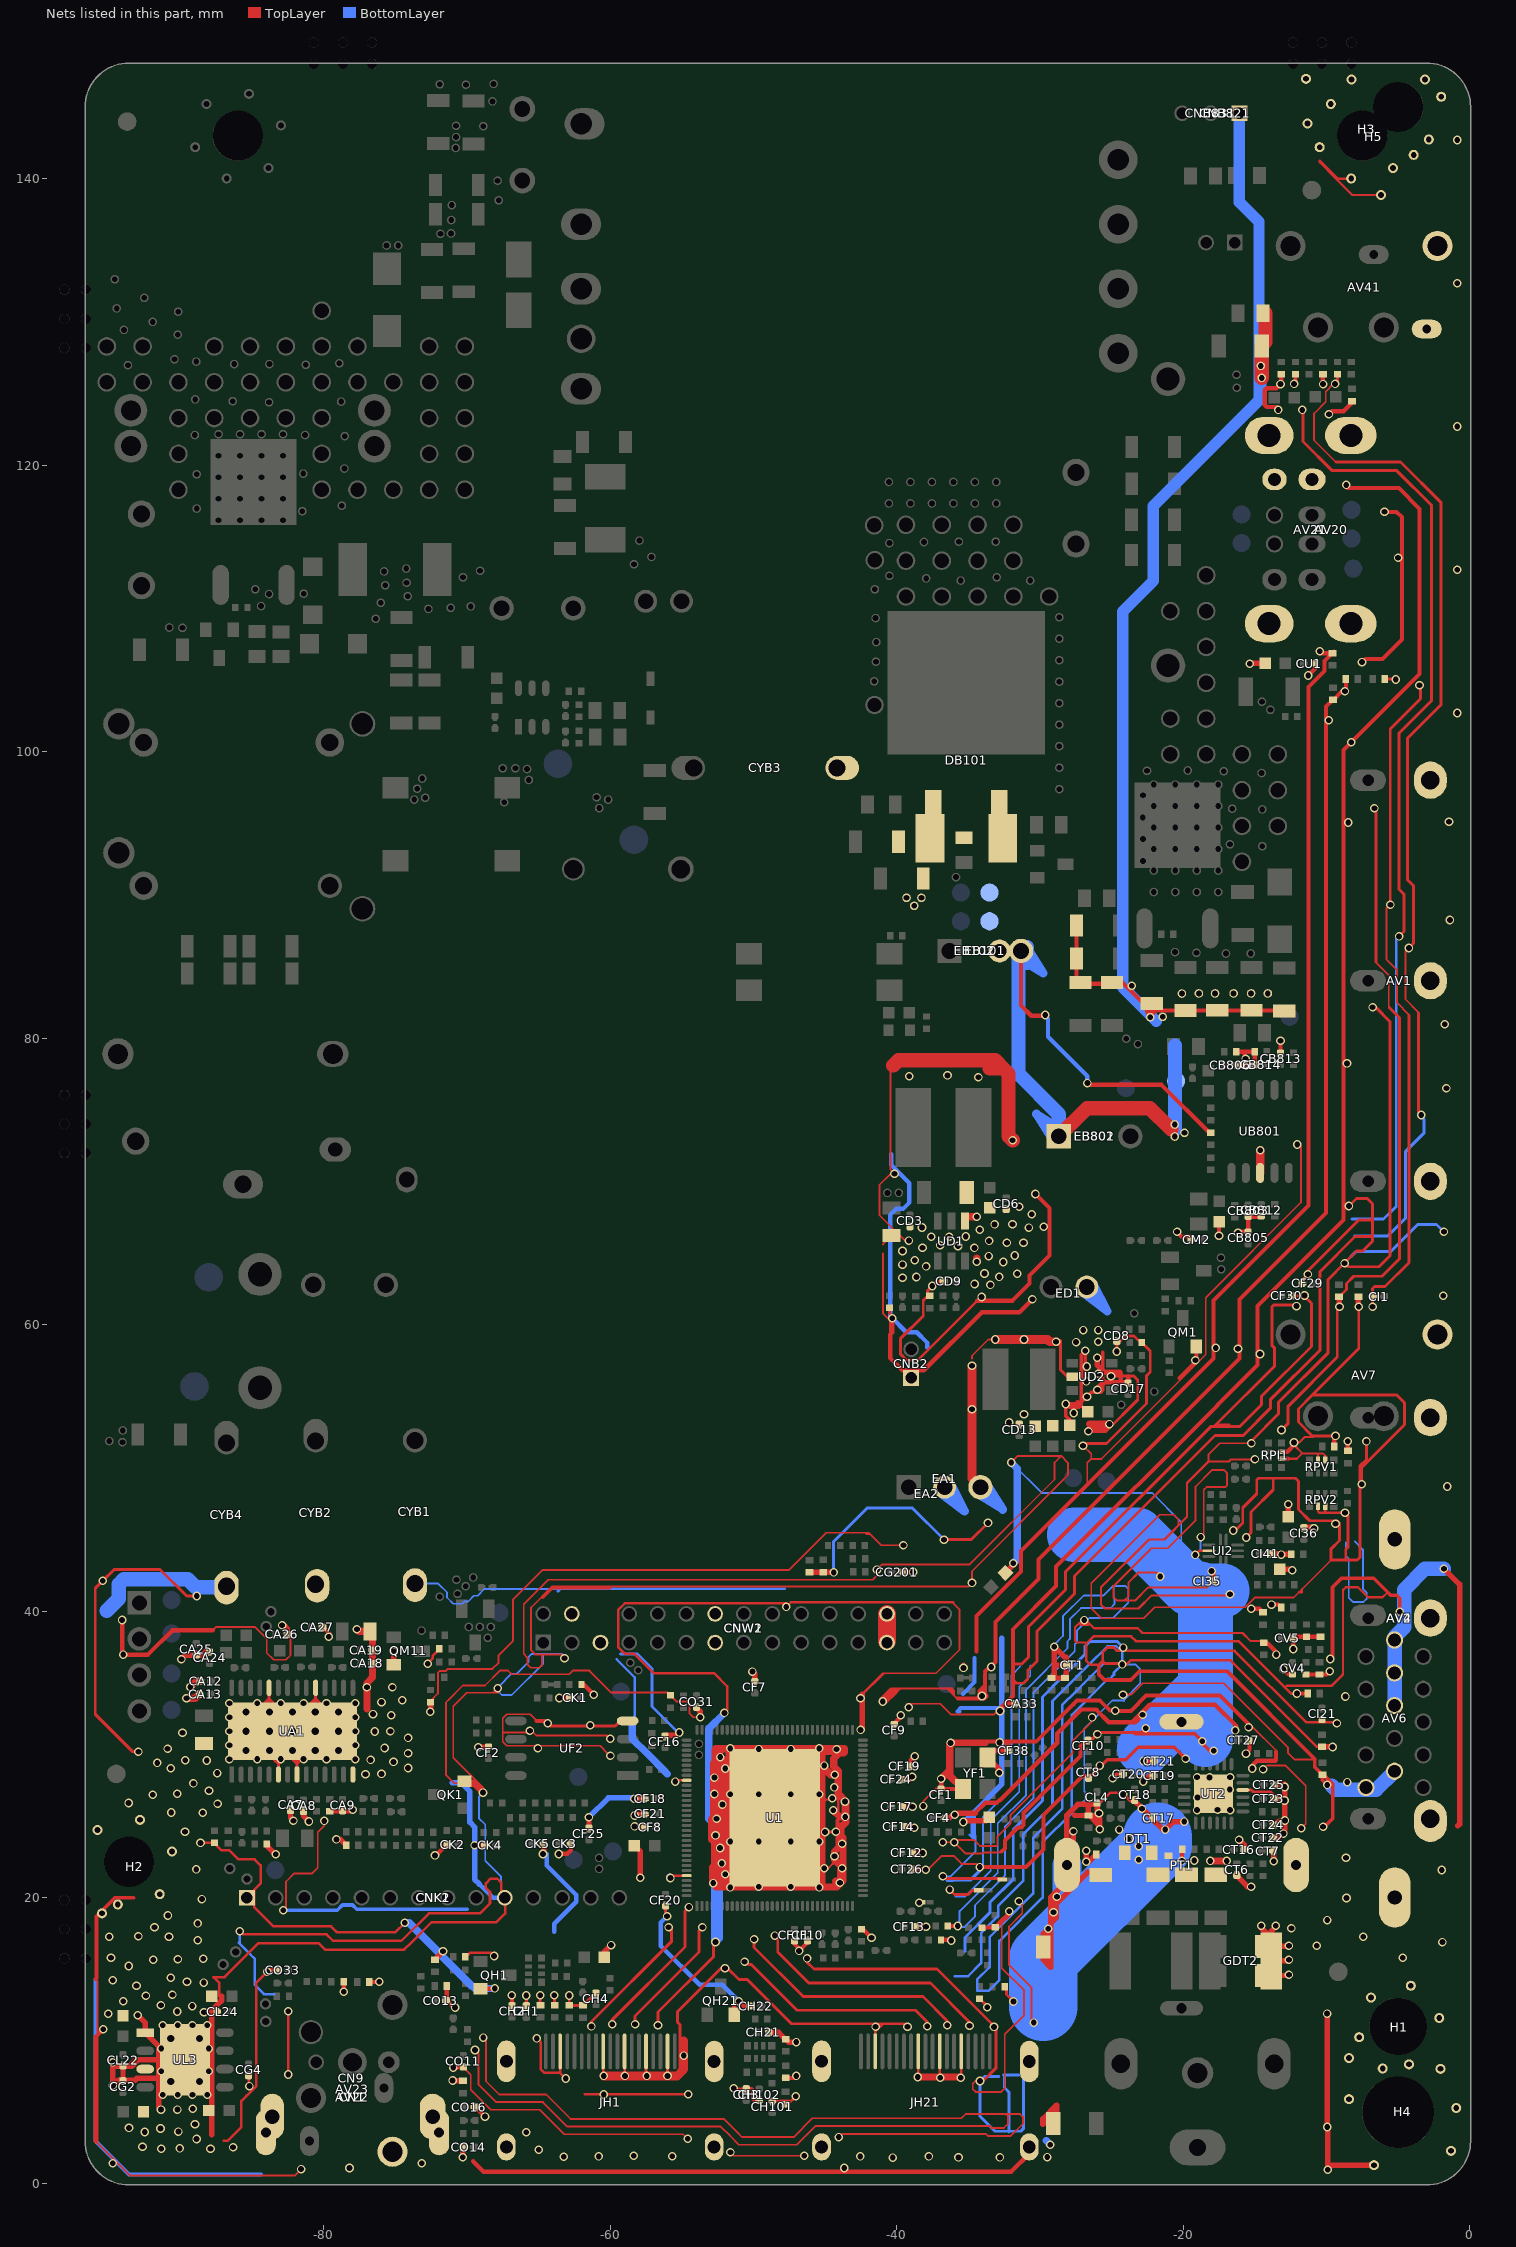
[diagram p0: the nets of this part, all layers, seen from the top]
# Altium PCB MISC86372.PcbDoc (part 9 of 16)
Units mm, origin at the board's own origin, x right, y up, seen from the top; angles counter-clockwise.
Board outline 96.73 x 148.13 mm, 2 copper layers (TopLayer, BottomLayer), stack 1.571 mm thick; 578 components, 318 nets, 2702 pads, 836 vias.

## Via types
v1: diameter 0.6, hole 0.4, TopLayer to BottomLayer, tented both sides, 816 vias
v2: diameter 0.7, hole 0.5, TopLayer to BottomLayer, tented both sides, 15 vias
v3: diameter 0.8, hole 0.5, TopLayer to BottomLayer, tented both sides, 5 vias

## Nets (pads, with @x,y where several pads share a name; then routed paths per layer and width w, separated by ;. In a path a pad name is that pad's centre, name@x,y a point inside that pad or via, vN(x,y) a via of type N, cw(c..) or ccw(c..) an arc to the next point about the centre after c; other vN are vias at no path point) (continued)
GND: (continued)
  TopLayer w0.203: v1(-92.943,30.175) -93.339,30.175 -95.953,32.79 -95.953,41.588 v1(-95.428,42.113) -94.634,42.907 -91.427,42.907 -89.566,41.046 v1(-88.875,41.046) ; UA1.EPAD@-84.277,33.426 -83.822,33.882 ; UA1.EPAD@-83.822,33.236 UA1.24@-83.822,34.661 ; -83.822,33.885 UA1.EPAD@-83.541,33.604 ; UA1.EPAD@-83.453,29.618 -83.172,29.337 ; UA1.6@-83.172,28.561 UA1.EPAD@-83.172,30.636 ; -83.172,29.34 UA1.EPAD@-82.716,29.796 ; UA1.EPAD@-82.153,29.618 -81.872,29.337 ; UA1.8@-81.872,28.561 UA1.EPAD@-81.872,29.964 ; -81.872,29.34 UA1.EPAD@-81.416,29.796 ; UA1.EPAD@-81.027,33.426 -80.572,33.882 ; UA1.EPAD@-80.572,33.28 UA1.19@-80.572,34.661 ; -80.572,33.885 UA1.EPAD@-80.291,33.604 ; CH1.2@-65.862,12.469 v1(-65.862,13.157) ; DH3.A@-64.897,12.495 v1(-64.897,13.183) ; -64.719,40.945 -64.072,41.593 ; v1(-64.364,32.156) -64.19,31.982 -62.357,31.982 ; -63.979,41.685 -64.072,41.593 ; v1(-63.906,13.183) -63.881,13.157 DH2.A@-63.881,12.49 ; v1@-62.865,13.047 v1(-62.865,13.157) DH81.A@-62.865,12.465 DH1.A@-61.906,12.465 DH1.A@-61.925,12.484 ; v1(-61.403,32.028) -61.449,31.982 -62.357,31.982 ; v1@-61.361,32.053 v1@-61.289,31.982 ; v1(-61.316,10.998) -61.316,11.341 -55.715,16.942 -55.715,17.912 -55.735,17.932 v1(-55.931,17.932) ; -59.999,41.593 -64.072,41.593 ; v1@-59.828,11.19 v1(-59.868,11.151) -59.868,11.46 -54.775,16.553 -54.775,19.063 v1(-54.508,19.329) ; -59.518,32.122 -59.657,31.982 -62.357,31.982 ; v1(-58.268,11.151) -58.268,11.731 -53.81,16.189 -53.81,17.678 v1(-53.569,17.919) ; v1@-56.629,11.112 v1(-56.667,11.074) -56.667,12.002 -52.782,15.888 -52.782,16.891 v1(-52.654,16.891) ; CF20.1@-56.138,19.388 -56.138,18.8 v1(-56.032,18.694) ; v1@-56,7.551 JH1.2@-56,9.258 ; -55.141,7.989 -55.141,11.122 -55.314,11.294 -55.314,12.026 -52.278,15.062 v1(-51.994,15.062) -51.807,15.062 -51.019,14.274 -50.437,14.274 -47.352,11.189 -42.139,11.189 ; v1(-51.381,6.688) -51.339,6.645 CH3.1@-50.588,6.645 ; v1(-50.622,15.508) -50.598,15.532 -50.545,15.532 -50.349,15.336 -50.17,15.336 -46.963,12.129 -38.699,12.128 -37.87,11.299 v1(-37.87,11.018) ; CH3.1@-50.506,6.669 -50.122,6.669 -50.057,6.604 -50.057,6.401 -50.053,6.397 -50.053,5.894 -49.957,5.798 CH102.1@-49.604,5.798 ; v1@-49.936,17.12 v1(-49.962,17.094) -49.962,16.511 -46.532,13.081 -38.167,13.081 -36.474,11.388 v1(-36.474,11.074) ; CH101.1@-48.819,5.81 -48.804,5.795 -48.142,5.795 -47.52,5.795 DH21.A@-47.738,5.577 ; v1(-48.509,17.34) -48.311,17.142 -48.311,16.189 -46.143,14.021 -37.652,14.021 -34.925,11.294 v1(-34.925,11.049) ; DH21.A@-47.904,5.557 -47.758,5.557 DH21.A@-47.738,5.577 ; DH21.A@-47.777,5.577 DH21.A@-47.738,5.577 ; v1(-47.05,6.133) -47.05,6.112 -47.585,5.577 DH21.A@-47.738,5.577 ; v1(-46.261,15.749) -46.279,15.731 -46.279,15.494 -45.783,14.999 -37.186,14.999 v1@-33.183,10.996 ; JH21.17@-41.5,9.258 -41.5,10.672 -40.983,11.189 -42.139,11.189 ; v1(-41.478,10.973) -41.262,11.189 ; RD5.1@-40.513,61.164 -40.513,60.782 -40.316,60.585 v1(-40.316,60.448) ; v1(-39.251,10.983) -39.456,11.189 -42.139,11.189 ; v1(-38.532,7.468) -38.5,7.499 JH21.11@-38.5,9.258 ; JH21.8@-37,9.258 -37,7.468 -37,7.46 v1(-36.957,7.417) ; CD9.1@-36.79,63.017 -37.186,63.017 v1(-37.516,62.687) -37.843,62.36 -37.843,61.995 -38.151,61.687 -38.151,60.604 -39.753,59.002 -39.753,57.963 -39.312,57.521 -38.523,57.521 -34.373,61.671 ; v1(-36.703,44.983) -34.798,44.983 v1(-33.63,46.152) ; v1@-36.662,21.605 v1(-36.779,21.488) -36.606,21.315 RA5.JP_2K@-32.63,21.315 ; v1@-36.424,11.1 v1@-36.424,11.269 ; v1(-36.297,20.553) -35.962,20.218 -35.013,20.218 -34.733,20.498 RA4.JP_2K@-34.28,20.498 ; v1@-35.535,7.366 -35.5,7.401 JH21.5@-35.5,9.258 ; RV5.1@-34.214,12.943 -33.68,12.41 v1(-33.68,12.344) ; v1(-34.188,7.188) -33.978,7.188 -33.058,8.108 ; -33.902,34.466 -33.927,34.466 -34.213,34.466 ; -33.864,35.179 -33.864,34.814 -33.902,34.776 -34.213,34.466 ; v1@-33.35,11.1 v1@-33.058,10.808 ; v1(-33.215,10.964) v1@-33.058,10.808 ; -33.058,8.153 v1@-33.058,10.808 ; RV3.1@-32.468,13.767 -32.339,13.638 -32.339,13.221 v1(-31.856,12.738) ; -31.902,35.204 -31.658,34.96 -31.153,34.96 -30.858,35.255 -30.858,35.844 -30.205,36.497 -30.205,38.592 -27.597,41.201 -27.597,42.445 -17.782,52.261 -15.813,52.261 -13.919,54.154 -13.919,54.747 -10.442,58.224 -10.442,63.707 -8.008,66.142 -7.645,66.142 ; -31.902,36.297 -31.268,36.297 -30.815,36.749 -30.815,38.883 -28.233,41.465 -28.233,42.715 -18.078,52.87 ; v1(-28.88,58.801) -28.578,58.499 ; -28.578,58.874 -28.578,56.842 -28.079,56.343 UD2.2@-27.74,56.343 ; v1(-27,51.537) -27,51.697 -25.366,51.697 -22.568,54.496 -22.568,56.426 -22.301,56.693 -22.301,58.159 RD8.2@-22.892,58.75 -22.98,58.75 -23.433,59.203 -24.051,59.203 -24.421,58.833 -24.638,58.833 v1@-24.638,58.141 ; v1(-26.619,52.553) -26.594,52.527 -25.399,52.527 -23.177,54.749 -23.177,56.128 -23.471,56.421 -24.361,56.421 -25.006,56.421 v1(-25.044,56.382) ; -25.705,55.666 -25.619,55.752 -25.474,55.896 ; v1(-25.155,53.051) v1@-24.874,53.051 ; -16.789,52.977 -17.741,52.977 ; v1(-16.51,45.618) -16.363,45.618 -15.845,46.136 -15.845,47.217 -14.869,48.192 -14.869,49.155 -14.756,49.268 -13.716,49.268 ; UT2.10@-15.832,27.504 -15.823,27.496 -15.227,27.496 -15.113,27.381 -14.356,27.381 -13.907,27.381 -13.625,27.099 CT23.1@-13.625,26.928 ; v1(-15.596,45.136) -15.261,45.471 -15.261,46.918 -13.716,48.463 -13.716,49.268 ; v1(-15.24,51.714) -15.24,51.866 -13.36,53.746 -13.36,54.547 -9.906,58.002 -9.906,63.119 v1(-8.738,64.287) ; v1(-13.142,52.638) -12.675,53.105 -12.675,54.299 -9.246,57.728 -9.246,61.138 v1@-9.119,61.265 ; CF30.2@-12.214,61.995 v1@-11.564,61.995 ; v1@-12.08,61.3 v1(-12.09,61.29) -12.09,61.366 -13.681,61.366 -13.818,61.23 -13.818,58.547 -13.615,58.344 -13.615,57.103 -17.741,52.977 ; CF29.2@-11.707,62.873 -11.707,63.096 v1(-11.294,63.509) -11.294,63.754 -7.742,67.305 -6.837,67.305 -6.782,67.361 ; v1(-11.684,123.85) -11.633,123.85 -11.633,121.642 -9.6,119.609 -5.093,119.609 -2.654,117.169 -2.654,103.569 -4.941,101.282 -4.941,90.387 -4.597,90.043 -4.597,87.431 v1(-4.932,87.096) ; v1(-11.532,62.027) v1@-11.564,61.995 ; v1@-10.251,125.669 v1(-10.236,125.654) ; -9.685,43.553 -7.856,43.553 -7.65,43.759 -7.65,50.135 -7.214,50.571 v1(-7.214,51.841) ; -9.673,43.566 -9.673,44.352 -9.096,44.929 -9.096,46.126 -9.271,46.302 -11.166,46.302 -11.95,47.085 -11.95,49.053 -12.165,49.268 -13.716,49.268 ; v1@-9.573,46.302 v1(-9.373,46.101) ; v1(-9.402,125.669) -9.298,125.669 -9.235,125.732 RA31.1@-9.235,126.346 ; v1(-9.373,52.222) -10.995,52.222 -11.963,53.191 -11.963,54.113 -10.983,55.093 ; -9.347,120.218 -4.841,120.218 ; DI2.A@-9.119,61.932 -8.606,62.444 -8.606,62.869 -8.103,63.373 -6.123,63.373 -4.902,64.594 -4.902,81.417 -5.613,82.128 ; v1(-8.707,46.853) -8.509,46.654 -8.509,44.446 -8.653,44.302 -8.653,44.281 -8.657,44.277 -8.657,43.553 ; v1(-8.433,68.275) -7.91,68.798 ; AV21.12@-8.3,122.07 AV21.12@-7.61,122.76 ; -7.849,66.142 -6.833,66.142 -6.782,66.192 ; v1(-7.747,61.239) -7.747,58.329 -10.983,55.093 ; v1(-7.544,48.844) -7.544,50.013 -4.547,53.01 -4.547,54.534 -5.105,55.093 -10.983,55.093 ; -7.417,68.798 -7.91,68.798 ; v1(-6.782,61.239) -6.775,61.246 CI1.2@-6.775,61.951 -6.782,61.957 -6.782,62.509 -6.636,62.655 -5.907,62.655 -4.242,64.32 -4.242,81.583 ; v1(-6.782,82.144) -6.563,82.144 -5.563,81.143 -5.563,64.795 -6.325,64.033 -8.484,64.033 v1(-8.738,64.287) ; v1(-6.655,96.037) -6.54,95.923 -6.54,85.324 ; DU1.A@-5.925,105.054 -5.182,105.054 v1(-5.156,105.029) ; -5.551,91.134 -5.551,91.415 ; v1(-5.537,89.306) -5.551,89.32 -5.551,91.415 ; -4.808,120.185 -4.841,120.218 ; v1(-4.247,86.287) -3.937,86.596 -3.937,90.642 -4.332,91.037 -4.332,100.958 -1.994,103.296 -1.994,117.371 -4.841,120.218 ; -3.581,81.748 -3.581,74.828 v1(-3.378,74.625) ; v1(-3.505,104.623) -3.429,104.546 -3.429,103.693 -5.551,101.571 -5.551,91.415 ; -34.404,33.934 -34.27,34.068 -34.27,34.122 -34.27,34.408 ; -34.404,33.934 -34.458,33.934 -35.806,33.934 -35.743,33.871 -34.521,33.871 -34.245,33.871 v1@-34.181,33.934 ; -34.404,33.934 v1@-34.181,33.934 ; -34.27,34.408 -34.127,34.265 -34.046,34.184 v1(-34.046,34.069) v1@-34.181,33.934 ; -34.27,34.408 -34.213,34.466 ; -18.078,52.87 -18.052,52.895 -17.822,52.895 -17.741,52.977 ; -18.078,52.87 -16.066,52.87 -14.529,54.407 -14.529,54.999 -11.051,58.476 -11.051,61.482 v1@-11.564,61.995 ; v1(-8.738,64.287) -7.899,65.126 -7.467,65.126 -6.782,65.811 -6.782,66.192 ; -7.91,68.798 -7.152,68.798 -6.782,68.428 -6.782,67.361 ; -6.782,66.192 -6.782,67.361
  TopLayer w0.229: v1@-60.5,7.589 v1@-60.5,7.592 ; v1@-57.5,7.589 JH1.5@-57.5,9.258 ; CT10.2@-26.645,31.007 -26.385,31.007 v1(-25.99,31.401) -25.868,31.524 -23.419,31.524 -22.915,31.524 v1(-22.619,31.82) ; v1@-25.808,29.112 -25.303,29.616 ; v1(-24.932,28.325) -24.932,28.366 -24.698,28.6 CT20.2@-24.254,28.6 ; -24.663,29.616 -25.303,29.616 ; -20.058,29.913 -20.631,30.486 -23.153,30.486 -24.023,29.616 -25.303,29.616 ; UT2.10@-15.832,27.504 UT2.10@-15.815,27.521
  TopLayer w0.254: -95.94,14.301 -95.869,14.372 -95.869,18.69 -94.576,19.983 -93.278,19.983 ; DH1.A@-61.906,12.465 -61.894,12.465 CH4.1@-61.006,13.353 ; CF5.1@-60.406,16.038 CF5.1@-60.406,15.824 CF5.1@-60.406,16.2 ; v1(-39.726,32.715) -39.726,32.562 CF9.1@-40.174,32.114 -40.174,32.191 v1@-39.675,32.69 ; CF1.1@-36.687,27.577 YF1.2@-35.369,27.577 ; CD10.1@-27.911,53.329 -28.194,53.612 v1(-28.194,54.454) ; -27.381,54.61 -27.33,54.559 -27.178,54.559 -27.178,54.305 -27.254,54.229 -27.969,54.229 v1(-28.194,54.454) ; -27.112,54.304 -27.112,54.574 ; v1(-26.764,56.027) -26.848,56.11 v1(-26.848,58.161) -27.112,57.897 -27.112,54.574 ; v1@-26.111,31.547 -26.111,31.54 v1@-26.094,31.558 ; -25.911,36.093 -25.911,35.603 -25.493,35.185 -23.666,35.185 -23.045,35.806 -16.95,35.806 -10.82,29.676 -10.82,29.114 -10.287,28.58 DV4.A@-10.287,28.556 ; -25.852,36.241 -25.616,36.477 ; -25.73,55.265 -26.421,55.265 v1(-26.72,54.966) -27.112,54.574 ; -25.619,55.417 -25.619,55.752 -25.619,55.859 -25.619,55.913 -25.619,56.772 -25.619,58.045 ; v1@-24.079,27.102 v1(-24.181,27.203) -24.152,27.203 -23.701,26.753 CT18.2@-23.393,26.753 ; -23.419,31.524 -23.334,31.439 -19.196,31.439 v1(-18.673,30.916) -18.83,30.916 -18.157,30.243 v1(-17.862,30.243) ; -20.058,29.913 v1(-19.837,29.693) ; v1(-13.032,35.954) -12.644,35.567 CV4.1@-12.37,35.567 ; RV6.1@-11.43,35.567 DV6.A@-10.49,35.567 -9.983,35.567 v1(-9.763,35.787) ; v1(-10.236,24.942) -10.135,24.942 -9.55,25.527 -9.55,27.897 -10.21,28.556 DV4.A@-10.287,28.556 ; v1(-9.946,27.858) -10.287,28.199 DV4.A@-10.287,28.556 ; v1(-9.728,36.652) -9.576,36.805 -9.576,41.665 -8.95,42.291 -6.706,42.291 -5.728,41.313 -5.524,41.11 -5.093,41.11 -4.877,40.894 v1(-4.877,39.954) ; AV6.16@-5.446,20 AV6.16@-5.227,20 ; v1(-28.194,54.454) -27.232,54.454 -27.112,54.574
  TopLayer w0.279: CF17.1@-39.58,26.34 -38.911,26.34 v1(-38.903,26.332) ; v1(-36.241,30.794) -36.161,30.874 -35.952,30.874 ; v1(-35.338,36.03) v1@-35.338,36.256 ; -34.417,37.177 -34.417,39.646 -31.319,42.744 -31.319,44.195 -27.331,48.183 ; v1(-34.215,22.123) -33.477,22.123 ; v1@-33.96,22.123 -33.477,22.123 ; -33.826,35.777 -33.51,36.092 v1@-33.459,36.092 ; v1@-33.495,36.056 v1@-33.459,36.092 ; v1@-33.403,36.092 v1@-33.459,36.092 ; v1(-32.821,30.819) v1@-32.876,30.874 ; v1(-32.791,33.02) -32.791,33.066 -32.33,33.528 ; v1@-32.756,33.229 -32.457,33.528 ; -32.672,23.216 -32.451,23.436 -32.451,23.98 -31.537,24.894 -31.294,24.894 ; -31.902,34.661 -31.902,34.309 ; CA33.1@-31.573,33.528 -32.33,33.528 ; -31.519,24.851 -31.475,24.894 -31.294,24.894 ; v1(-28.999,37.503) -28.956,37.46 DK3.A@-28.956,35.421 ; -27.675,33.475 -27.792,33.358 ; -27.318,48.196 -26.703,48.81 -17.889,57.625 v1@-17.889,58.42 ; CT10.2@-26.645,30.832 -26.916,30.832 -27.18,30.568 -27.18,29.869 -31.14,25.908 -31.14,25.048 -31.294,24.894 ; v1(-25.832,29.21) -25.808,29.186 -25.808,29.112 -26.442,28.478 CT8.1@-26.619,28.478 -27.027,28.478 -29.743,25.761 -29.743,23.361 -30.981,22.123 -33.477,22.123 ; v1@-24.689,33.02 -24.028,33.02 ; v1(-20.429,66.469) -20.141,66.181 -20.141,66.139 -19.478,66.139 CM2.1@-19.478,65.913 ; -20.26,56.267 -19.152,57.375 v1(-19.152,57.506) -19.088,57.569 QM1.E@-19.088,58.471 ; v1(-17.726,58.369) -17.838,58.369 v1@-17.889,58.42 ; -17.621,54.354 -28.881,43.094 -28.881,41.734 -31.902,38.712 -31.902,36.297 -31.902,35.204 -31.902,34.309 ; -17.607,54.368 -14.8,57.174 -14.8,59.106 ; v1(-16.18,58.318) v1@-16.078,58.42 ; v1(-15.439,31.885) -15.439,32.102 -17.424,34.087 -22.588,34.087 -23.655,33.02 -24.028,33.02 ; v1(-14.64,57.94) -14.8,58.101 -14.8,59.106 ; v1(-9.834,102.184) v1@-10.033,102.384 ; DU4.A@-9.459,106.985 -10.135,106.308 -10.135,105.613 -11.252,104.496 -11.252,68.3 -17.889,61.663 v1@-17.889,58.42 ; DU2.A@-8.655,105.054 -8.655,104.274 v1(-8.712,104.216) -8.92,104.216 -9.523,103.613 DU3.A@-9.55,103.613 -10.033,103.131 v1@-10.033,102.384 ; v1(-8.611,118.618) -8.534,118.542 -8.534,118.39 -4.947,118.39 -3.505,116.948 -3.505,105.423 v1(-8.28,100.648) -8.814,100.115 -8.814,67.29 -14.8,61.304 -14.8,59.106 ; v1(-7.518,106.248) -7.29,106.477 -6.08,106.477 -4.724,107.832 -4.724,116.36 -5.106,116.741 v1(-5.95,116.741) ; -35.952,30.874 -33.63,30.874 ; -35.952,30.874 -36.16,30.666 -36.16,30.577 -36.019,30.718 -33.785,30.718 -33.63,30.874 ; -33.63,30.874 v1@-32.876,30.874 ; v1@-33.459,36.092 -33.122,36.43 -33.122,39.217 -30.1,42.239 -30.1,43.599 -16.078,57.621 v1@-16.078,58.42 ; v1@-32.876,30.874 -30.277,30.874 -27.792,33.358 ; -32.457,33.528 -31.902,34.082 -31.902,34.309 ; -32.457,33.528 -32.33,33.528 ; -27.792,33.358 -27.406,33.744 -25.828,33.744 -25.13,33.045 v1(-24.74,33.045) -24.714,33.02 -24.028,33.02 ; v1@-16.078,58.42 -16.078,61.75 -10.033,67.795 v1@-10.033,102.384
  TopLayer w0.3: EB101.2@-31.323,86.081 -31.323,82.275 -30.607,81.559 v1@-29.642,81.559 ; RB822.2@-27.459,87.859 RB821.2@-27.459,85.547 -27.459,84.077 -27.178,83.796 -24.867,83.796 -24.79,83.872 -24.245,83.872 -22.291,81.918 -22.271,81.918 -13.06,81.918 RB818.2@-13.03,81.888 ; v1(-26.692,76.857) -26.568,76.733 -24.663,76.733 ; v1@-26.518,76.733 -24.663,76.733 ; RB134.1@-18.085,73.399 -18.182,73.399 -21.516,76.733 -24.663,76.733 ; v1(-17.501,66.192) CB801.2@-17.501,67.188 ; CB806.2@-16.41,78.105 -16.235,78.105 -15.248,78.105 CB814.2@-15.223,78.13 ; RB803.1@-16.231,79.045 -15.729,79.045 ; v1(-16.18,66.396) -16.106,66.469 CB805.1@-15.469,66.469 CB803.2@-15.469,67.52 CB812.1@-14.58,67.52 ; v1(-15.646,78.562) -15.729,78.645 -15.729,79.045 ; RB833.1@-15.223,79.041 -15.227,79.045 -15.729,79.045 ; CB814.2@-15.005,78.13 RB833.1@-15.005,79.045 ; CB813.1@-13.208,78.812 v1@-13.208,79.807 ; v1@-10.251,125.669 DA31.A@-10.251,126.346
  TopLayer w0.305: -95.91,2.989 -95.91,10.287 v1(-95.402,10.795) ; v1(-94.082,39.37) -94.082,37.033 v1(-94.005,36.957) -92.278,36.957 -90.588,38.648 -87.757,38.648 ; v1(-83.957,14.808) -83.83,14.935 CO33.1@-83.28,14.935 ; v1(-82.912,39.01) -82.732,39.01 -82.502,38.78 CA26.1@-82.502,38.372 ; CA27.2@-80.038,38.869 -79.603,38.434 -79.603,38.253 v1(-79.654,38.202) ; RA11.1@-79.668,26.023 RA11.1@-79.588,26.023 ; RA11.1@-79.582,26.018 CA9.1@-78.677,26.018 ; RO4.1@-78.62,14.118 -78.62,13.418 v1(-78.613,13.411) ; v1(-77.987,26.119) -78.083,26.023 CA9.1@-78.689,26.023 -78.04,26.023 v1@-77.978,26.086 ; DI9.A@-76.816,14.101 -76.145,14.101 v1(-76.124,14.122) ; v1(-72.238,22.936) -72.177,22.936 CK2.1@-71.425,23.688 ; DI6.A@-71.406,13.818 CO13.1@-71.406,12.802 -70.929,12.324 v1(-70.835,12.324) ; v1(-70.968,8.128) -70.961,8.135 CO11.1@-70.256,8.135 ; -69.571,1.575 -68.847,0.851 -32.017,0.851 -30.75,2.118 JH21.23@-30.75,2.59 ; CO16.1@-69.425,5.371 -68.76,4.705 v1(-68.747,4.705) ; v1(-69.215,30.496) -69.197,30.514 CF2.1@-68.504,30.514 ; QH1.E@-69.063,13.627 -68.089,13.627 v1(-68.062,13.654) ; v1(-66.878,13.176) -66.861,13.158 CH2.2@-66.861,12.474 ; -65.134,32.325 -64.618,32.325 -64.449,32.156 v1(-64.364,32.156) ; v1(-63.602,23.038) -63.593,23.047 -63.009,23.047 -62.745,23.31 CK3.1@-62.745,23.749 ; RF13.2@-62.008,34.87 -61.852,34.87 -61.159,34.177 v1(-61.159,34.161) ; QH21.E@-51.333,11.811 -51.333,12.476 v1@-51.046,12.763 ; v1(-51.033,12.763) v1@-51.046,12.763 ; CH22.2@-50.078,12.421 -50.704,12.421 v1@-51.046,12.763 ; DH22.A@-47.904,7.38 DH22.A@-47.611,7.38 ; DH22.A@-47.752,7.403 -47.157,7.403 v1(-47.015,7.544) ; CF11.2@-47.14,16.95 -47.14,16.762 -46.821,16.442 v1(-46.821,16.273) -46.226,16.867 CF10.1@-46.226,16.95 ; RF16.2@-42.469,17.799 -42.368,17.799 v1(-41.766,17.197) ; v1(-40.316,60.448) -40.316,59.445 -40.464,59.297 -40.464,57.668 -39.607,56.81 -38.11,56.81 -34.054,60.865 -31.438,60.865 v1(-30.531,61.773) ; CF19.2@-39.021,29.159 -39.021,29.581 v1(-38.741,29.862) ; CF12.1@-38.869,23.114 -38.202,23.114 v1(-38.192,23.103) ; CT26.1@-38.844,21.971 -38.001,21.971 v1(-37.975,21.945) ; RF12.2@-36.913,17.043 v1@-36.251,17.043 ; CF1.1@-36.906,27.603 v1(-36.906,28.296) ; RO1.1@-36.43,18.009 v1(-35.738,18.009) ; v1@-36.236,17.028 v1@-36.251,17.043 ; v1(-36.194,16.997) -36.241,17.043 v1@-36.251,17.043 ; -34.533,25.895 -33.825,26.604 -33.82,26.604 -33.032,26.604 -32.865,26.771 -32.815,26.771 -28.79,30.797 -28.79,31.448 -27.116,33.122 -26.086,33.122 -25.202,32.237 ; -34.373,61.671 -31.924,61.671 -30.734,62.861 -30.734,63.427 -29.337,64.824 -29.337,68.128 v1(-30.32,69.111) ; RV1.1@-34.043,17.903 -33.133,17.903 RI1.1@-33.122,17.914 -32.664,18.371 -32.214,18.821 v1@-32.156,18.821 ; v1(-25.99,55.448) -25.99,55.488 -25.619,55.859 -25.506,55.972 -24.361,55.972 ; -24.436,56.675 -24.361,56.599 -24.361,56.421 -24.361,55.972 ; CD17.1@-23.849,55.95 CD17.1@-23.849,55.972 ; -23.849,56.38 CD17.1@-23.849,55.972 ; -23.558,32.237 -22.33,33.465 -17.78,33.465 -16.281,31.966 -16.281,31.75 -16.366,31.665 v1(-16.37,31.665) ; -23.376,32.237 -25.202,32.237 ; v1(-22.836,32.75) -23.349,32.237 -25.202,32.237 ; v1(-22.784,28.092) -22.372,28.504 CT19.1@-22.116,28.504 ; v1@-22.753,29.515 CT21.1@-22.091,29.515 ; v1(-20.091,22.555) -20.085,22.562 LT5.2@-20.085,23.368 ; CI35.2@-17.91,42.088 v1@-17.91,42.677 ; v1(-15.621,30.048) -15.628,30.055 -15.374,30.309 CT27.1@-15.374,30.963 ; v1(-15.251,40.157) -14.681,40.157 DV2.A@-14.427,39.903 ; v1(-15.189,29.007) -15.189,29.21 -14.862,29.537 -13.558,29.537 -13.523,29.572 -13.523,30.177 ; DI1.A@-14.385,37.8 -14.363,37.8 -14.173,37.8 -13.514,37.141 v1(-13.514,36.957) ; v1(-13.836,40.452) -13.376,40.452 DV1.A@-13.158,40.234 ; CT24.1@-13.647,25.07 -13.342,25.375 v1(-12.903,25.375) ; v1(-13.36,123.85) -13.36,123.927 -13.494,124.06 -14.166,124.06 -14.314,124.209 -14.314,125.219 -14.166,125.368 -13.494,125.368 v1(-13.208,125.654) -13.157,125.705 DA32.A@-13.157,126.346 ; RPI1.3@-13.139,50.626 -12.7,50.626 ; RPI1.5@-13.139,51.126 -12.729,51.126 -12.268,51.587 v1(-12.268,51.765) ; v1(-12.314,37.347) CV5.1@-12.314,38.093 -12.199,38.208 DV7.A@-10.431,38.208 ; v1(-12.263,125.669) -12.167,125.765 RA32.1@-12.167,126.346 ; v1(-12.065,34.239) DV3.A@-11.322,34.239 ; v1(-11.278,105.308) -10.772,105.814 CU1.2@-10.772,106.147 ; v1(-10.465,107) -10.341,106.876 DU4.A@-9.576,106.876 ; DV8.A@-9.456,51.486 -9.456,52.139 v1(-9.373,52.222) ; DV9.A@-8.509,51.174 -8.509,51.85 v1(-8.507,51.852) ; DA33.A@-8.23,124.469 -8.23,124.337 -8.797,123.769 -9.55,123.769 ; -24.361,55.972 CD17.1@-23.849,55.972 ; -9.55,123.769 -9.768,123.551 v1(-9.83,123.551) -9.612,123.769 -9.55,123.769